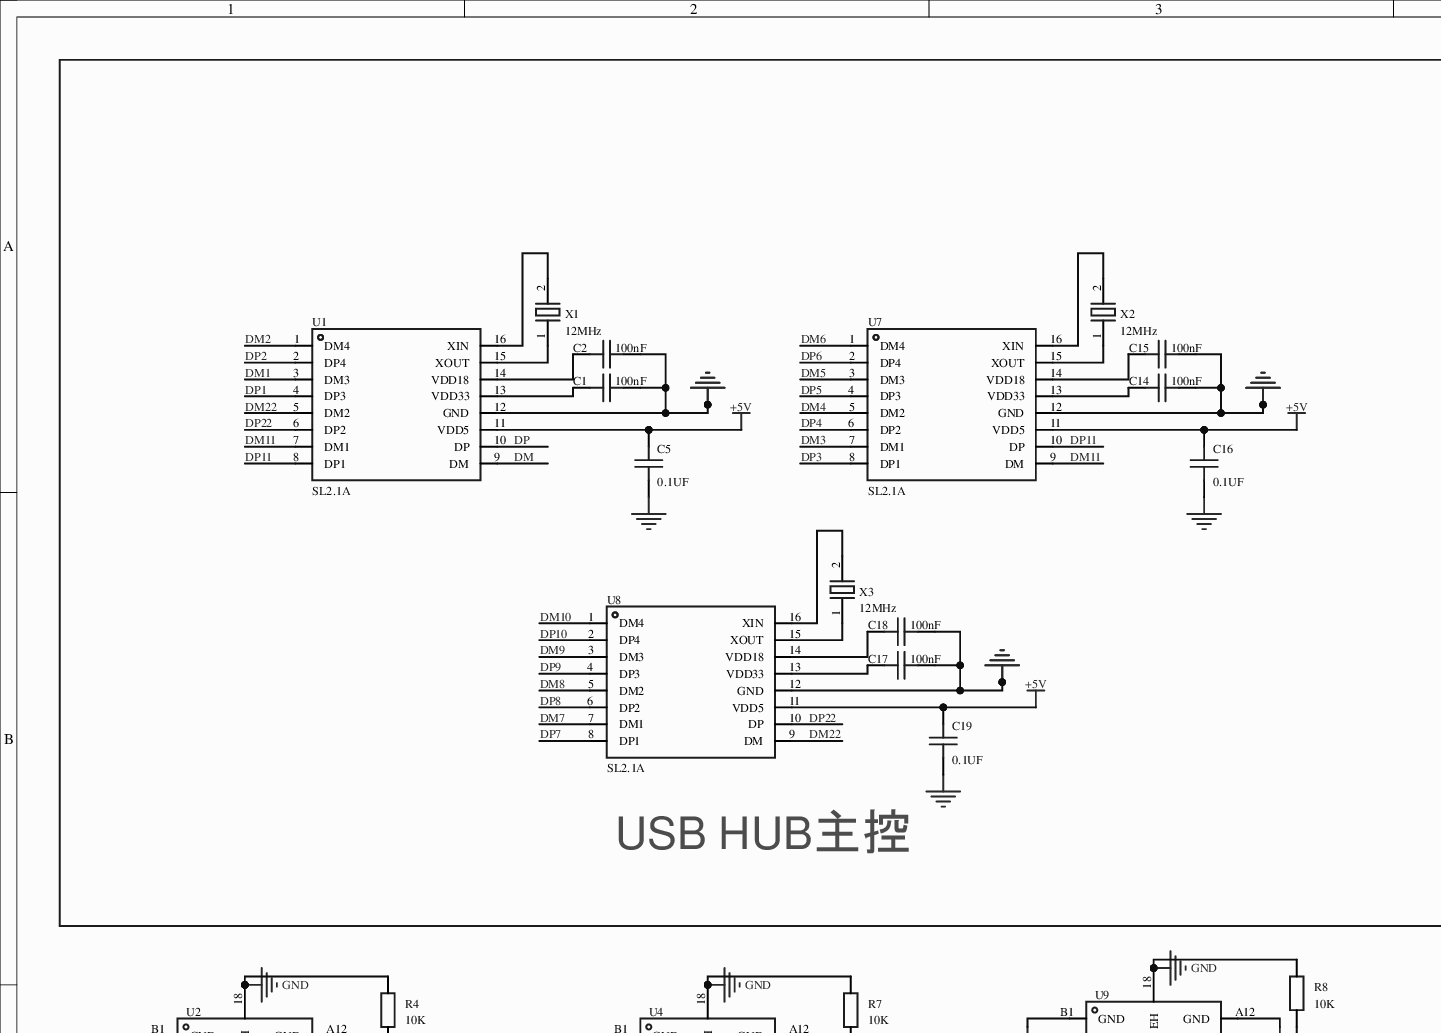
[diagram p0: MISC51596-3.schdoc, top left]
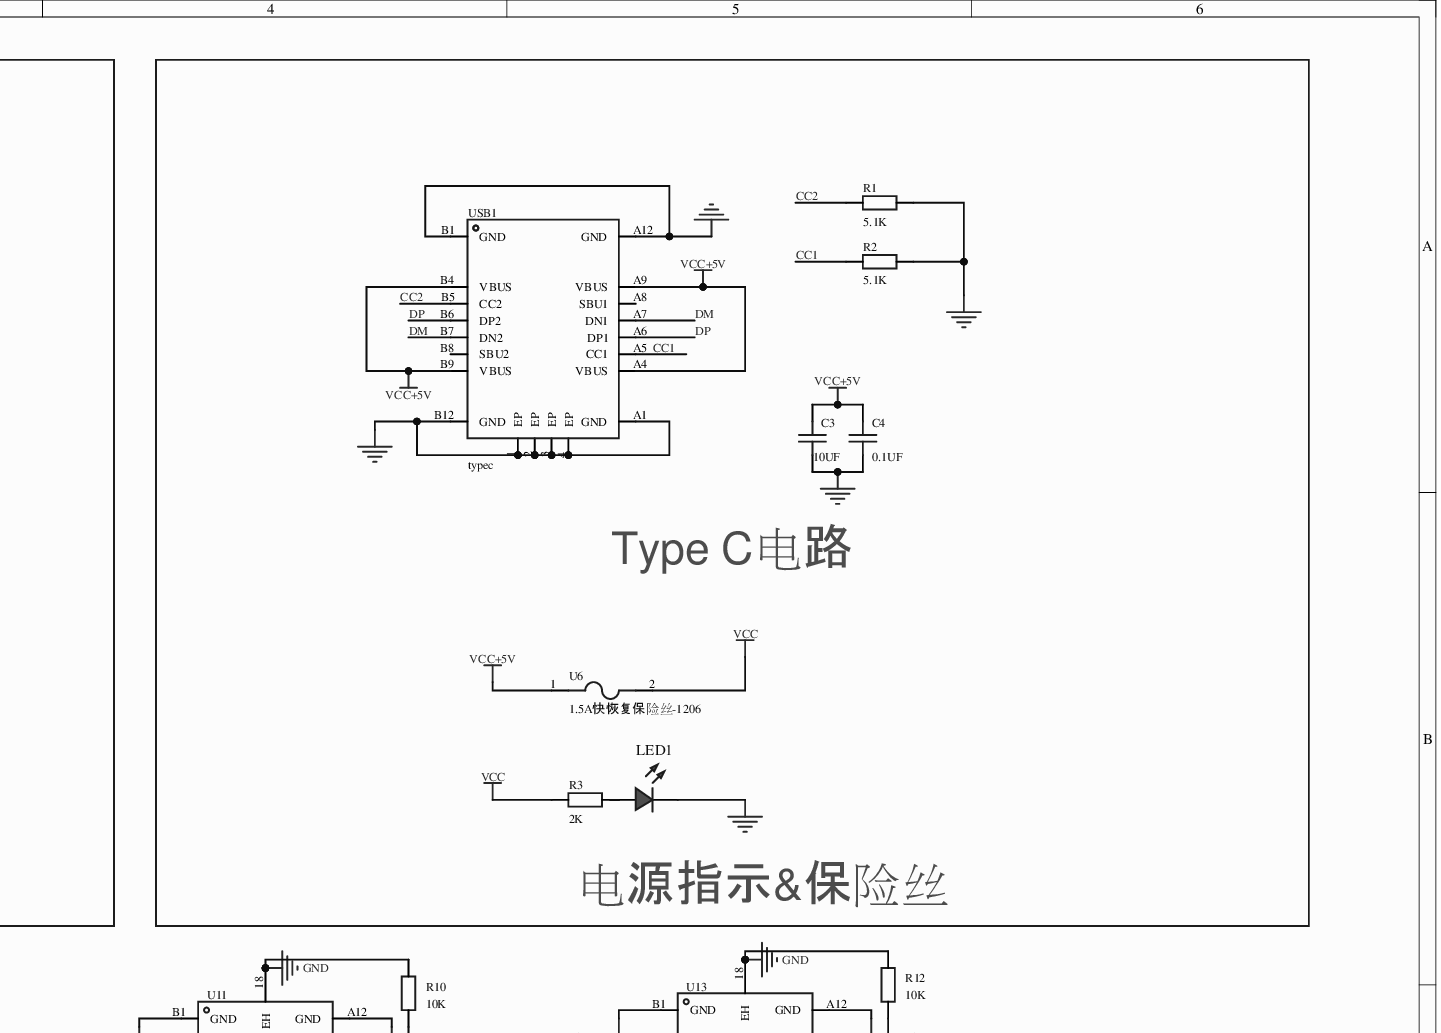
[diagram p1: MISC51596-3.schdoc, top right]
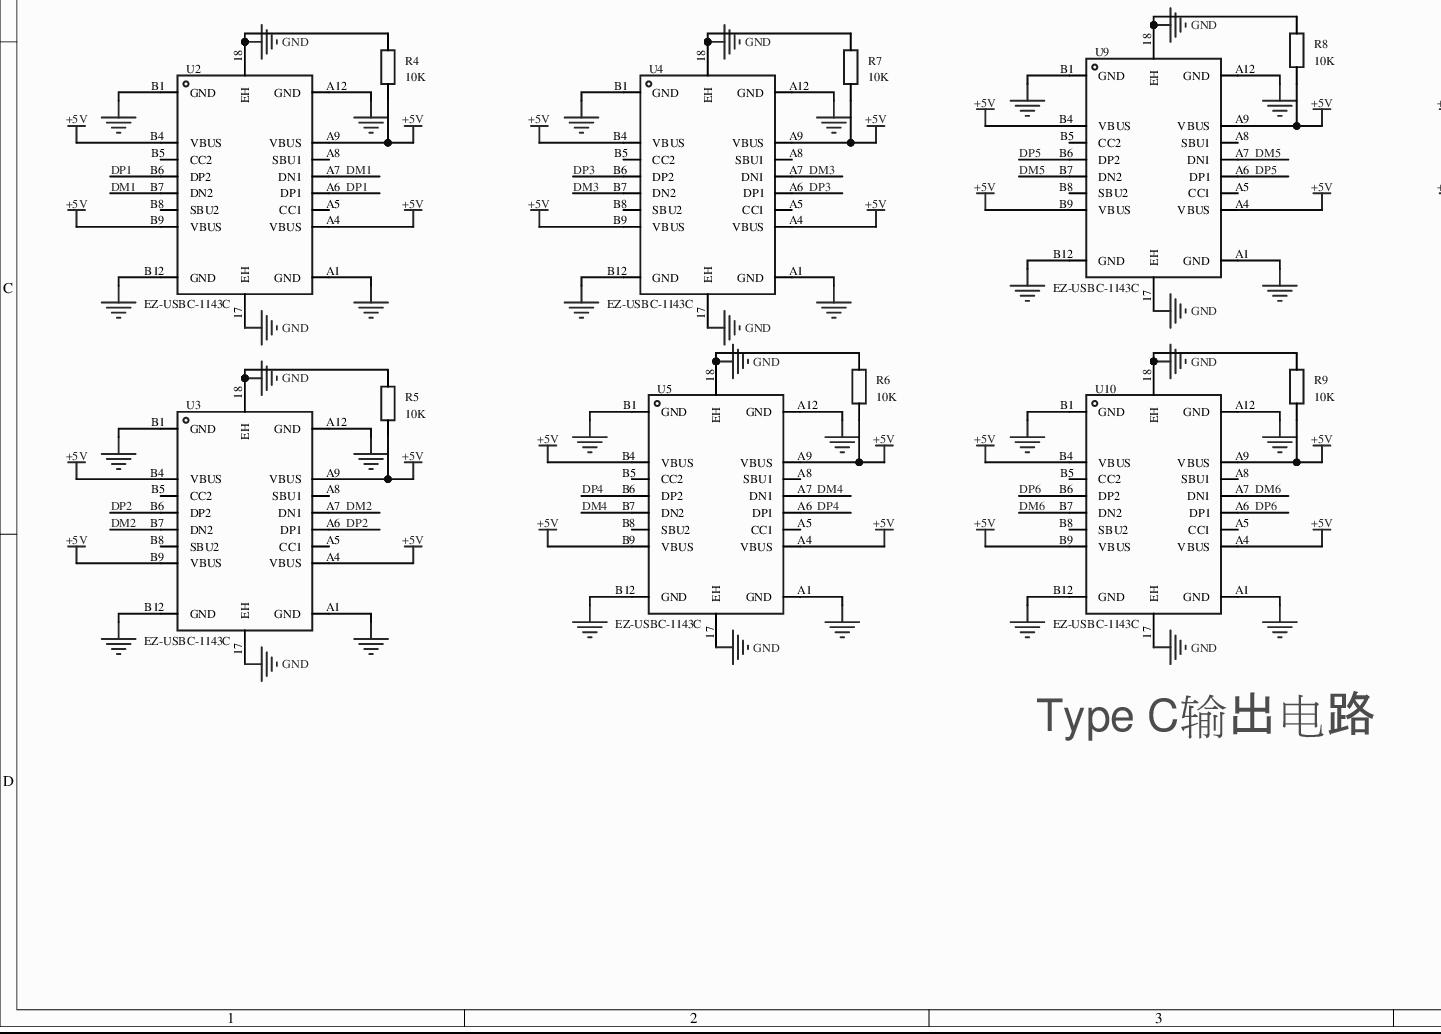
[diagram p2: MISC51596-3.schdoc, bottom left]
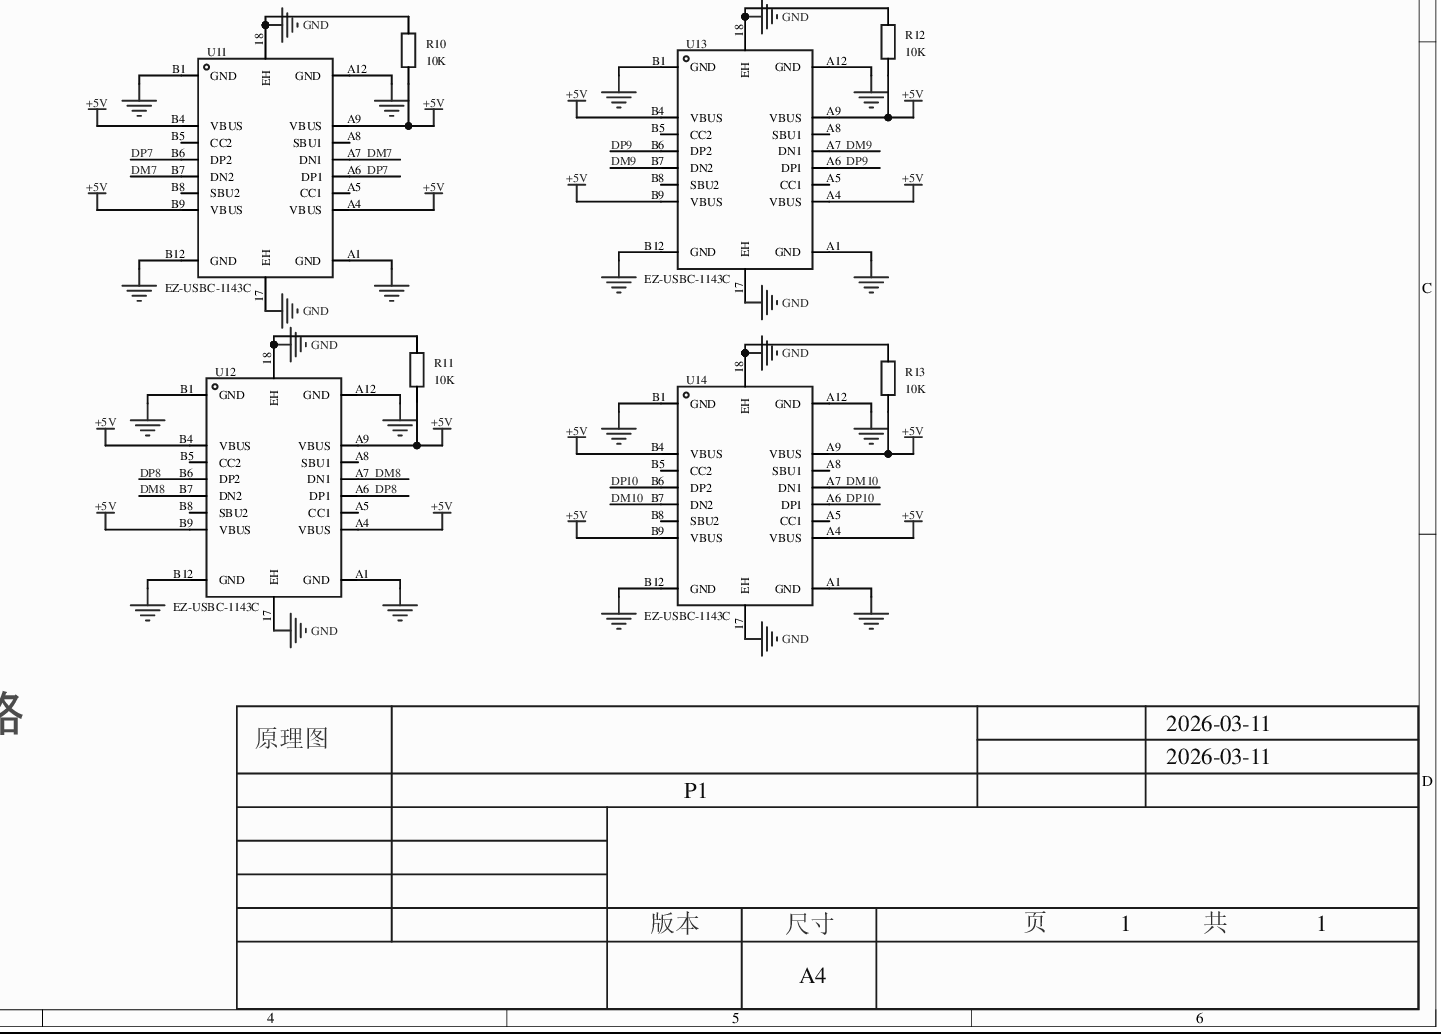
[diagram p3: MISC51596-3.schdoc, bottom right]
# Altium project MISC51596-2.PrjPcb
1 sheet, 43 parts. Net scope: global (net labels, ports and power ports of the same name join across sheets).
Board file: MISC51596.pcbdoc

## Sheet MISC51596-3.schdoc
size 420 x 297 mm; Version: V1.0; @Project Name: MISC51596; @Page Count: 1; @Update Date: 2026-03-11; @Create Date: 2026-03-11; @Schematic Name: MISC51596; @Page No: 1

### Parts
C1  100nF  [C0805]
C2  100nF  [C0805]
C3  10UF  [C0805]
C4  0.1UF  [C0805]
C5  0.1UF  [C0805]
C14  100nF  [C0805]
C15  100nF  [C0805]
C16  0.1UF  [C0805]
C17  100nF  [C0805]
C18  100nF  [C0805]
C19  0.1UF  [C0805]
LED1  (no value)  [LED_0805]
R1  5.1K  [R0805]
R2  5.1K  [R0805]
R3  2K  [R0805]
R4  10K  [R0603]
R5  10K  [R0603]
R6  10K  [R0603]
R7  10K  [R0603]
R8  10K  [R0603]
R9  10K  [R0603]
R10  10K  [R0603]
R11  10K  [R0603]
R12  10K  [R0603]
R13  10K  [R0603]
U1  SL2.1A  [SOP-16_L10.0-W3.9-P1.27-LS6.0-BL]
U2  EZ-USBC-1143C  [USB-SMD_EZ-USBC-1143C]
U3  EZ-USBC-1143C  [USB-SMD_EZ-USBC-1143C]
U4  EZ-USBC-1143C  [USB-SMD_EZ-USBC-1143C]
U5  EZ-USBC-1143C  [USB-SMD_EZ-USBC-1143C]
U6  1.5A快恢复保险丝-1206  [F1206]
U7  SL2.1A  [SOP-16_L10.0-W3.9-P1.27-LS6.0-BL]
U8  SL2.1A  [SOP-16_L10.0-W3.9-P1.27-LS6.0-BL]
U9  EZ-USBC-1143C  [USB-SMD_EZ-USBC-1143C]
U10  EZ-USBC-1143C  [USB-SMD_EZ-USBC-1143C]
U11  EZ-USBC-1143C  [USB-SMD_EZ-USBC-1143C]
U12  EZ-USBC-1143C  [USB-SMD_EZ-USBC-1143C]
U13  EZ-USBC-1143C  [USB-SMD_EZ-USBC-1143C]
U14  EZ-USBC-1143C  [USB-SMD_EZ-USBC-1143C]
USB1  typec  [USB-C-SMD_KH-TYPE-C-16P]
X1  12MHz  [CRYSTAL-SMD_L11.1-W4.8-LS12.3]
X2  12MHz  [CRYSTAL-SMD_L11.1-W4.8-LS12.3]
X3  12MHz  [CRYSTAL-SMD_L11.1-W4.8-LS12.3]

### Blocks framed on the sheet
USB HUB主控: C1 C2 C5 C14-C19 U1 U7 U8 X1-X3

### Nets
+5V: C5.2 C16.2 C19.2 R4.1 R5.1 R6.1 R7.1 R8.1 R9.1 R10.1 R11.1 R12.1 R13.1 U1.11(VDD5) U2.A4(VBUS) U2.A9(VBUS) U2.B4(VBUS) U2.B9(VBUS) U3.A4(VBUS) U3.A9(VBUS) U3.B4(VBUS) U3.B9(VBUS) U4.A4(VBUS) U4.A9(VBUS) U4.B4(VBUS) U4.B9(VBUS) U5.A4(VBUS) U5.A9(VBUS) U5.B4(VBUS) U5.B9(VBUS) U7.11(VDD5) U8.11(VDD5) U9.A4(VBUS) U9.A9(VBUS) U9.B4(VBUS) U9.B9(VBUS) U10.A4(VBUS) U10.A9(VBUS) U10.B4(VBUS) U10.B9(VBUS) U11.A4(VBUS) U11.A9(VBUS) U11.B4(VBUS) U11.B9(VBUS) U12.A4(VBUS) U12.A9(VBUS) U12.B4(VBUS) U12.B9(VBUS) U13.A4(VBUS) U13.A9(VBUS) U13.B4(VBUS) U13.B9(VBUS) U14.A4(VBUS) U14.A9(VBUS) U14.B4(VBUS) U14.B9(VBUS)
GND: C1.2 C2.2 C3.1 C4.1 C5.1 C14.2 C15.2 C16.1 C17.2 C18.2 C19.1 LED1.1(C) R1.2 R2.2 R4.2 R5.2 R6.2 R7.2 R8.2 R9.2 R10.2 R11.2 R12.2 R13.2 U1.12(GND) U2.17(EH) U2.18(EH) U2.A1(GND) U2.A12(GND) U2.B1(GND) U2.B12(GND) U3.17(EH) U3.18(EH) U3.A1(GND) U3.A12(GND) U3.B1(GND) U3.B12(GND) U4.17(EH) U4.18(EH) U4.A1(GND) U4.A12(GND) U4.B1(GND) U4.B12(GND) U5.17(EH) U5.18(EH) U5.A1(GND) U5.A12(GND) U5.B1(GND) U5.B12(GND) U7.12(GND) U8.12(GND) U9.17(EH) U9.18(EH) U9.A1(GND) U9.A12(GND) U9.B1(GND) U9.B12(GND) U10.17(EH) U10.18(EH) U10.A1(GND) U10.A12(GND) U10.B1(GND) U10.B12(GND) U11.17(EH) U11.18(EH) U11.A1(GND) U11.A12(GND) U11.B1(GND) U11.B12(GND) U12.17(EH) U12.18(EH) U12.A1(GND) U12.A12(GND) U12.B1(GND) U12.B12(GND) U13.17(EH) U13.18(EH) U13.A1(GND) U13.A12(GND) U13.B1(GND) U13.B12(GND) U14.17(EH) U14.18(EH) U14.A1(GND) U14.A12(GND) U14.B1(GND) U14.B12(GND) USB1.1(EP) USB1.2(EP) USB1.3(EP) USB1.4(EP) USB1.A1(GND) USB1.A12(GND) USB1.B1(GND) USB1.B12(GND)
VCC: R3.2 U6.2
VCC+5V: C3.2 C4.2 U6.1 USB1.A4(VBUS) USB1.A9(VBUS) USB1.B4(VBUS) USB1.B9(VBUS)
CC1: R2.1 USB1.A5(CC1)
CC2: R1.1 USB1.B5(CC2)
DM: U1.9(DM) USB1.A7(DN1) USB1.B7(DN2)
DM1: U1.3(DM3) U2.A7(DN1) U2.B7(DN2)
DM2: U1.1(DM4) U3.A7(DN1) U3.B7(DN2)
DM3: U4.A7(DN1) U4.B7(DN2) U7.7(DM1)
DM4: U5.A7(DN1) U5.B7(DN2) U7.5(DM2)
DM5: U7.3(DM3) U9.A7(DN1) U9.B7(DN2)
DM6: U7.1(DM4) U10.A7(DN1) U10.B7(DN2)
DM7: U8.7(DM1) U11.A7(DN1) U11.B7(DN2)
DM8: U8.5(DM2) U12.A7(DN1) U12.B7(DN2)
DM9: U8.3(DM3) U13.A7(DN1) U13.B7(DN2)
DM10: U8.1(DM4) U14.A7(DN1) U14.B7(DN2)
DM11: U1.7(DM1) U7.9(DM)
DM22: U1.5(DM2) U8.9(DM)
DP: U1.10(DP) USB1.A6(DP1) USB1.B6(DP2)
DP1: U1.4(DP3) U2.A6(DP1) U2.B6(DP2)
DP2: U1.2(DP4) U3.A6(DP1) U3.B6(DP2)
DP3: U4.A6(DP1) U4.B6(DP2) U7.8(DP1)
DP4: U5.A6(DP1) U5.B6(DP2) U7.6(DP2)
DP5: U7.4(DP3) U9.A6(DP1) U9.B6(DP2)
DP6: U7.2(DP4) U10.A6(DP1) U10.B6(DP2)
DP7: U8.8(DP1) U11.A6(DP1) U11.B6(DP2)
DP8: U8.6(DP2) U12.A6(DP1) U12.B6(DP2)
DP9: U8.4(DP3) U13.A6(DP1) U13.B6(DP2)
DP10: U8.2(DP4) U14.A6(DP1) U14.B6(DP2)
DP11: U1.8(DP1) U7.10(DP)
DP22: U1.6(DP2) U8.10(DP)
NetC1_1: C1.1 U1.13(VDD33)
NetC2_1: C2.1 U1.14(VDD18)
NetC14_1: C14.1 U7.13(VDD33)
NetC15_1: C15.1 U7.14(VDD18)
NetC17_1: C17.1 U8.13(VDD33)
NetC18_1: C18.1 U8.14(VDD18)
NetLED1_2: LED1.2(A) R3.1
NetU1_15: U1.15(XOUT) X1.1
NetU1_16: U1.16(XIN) X1.2(GND)
NetU7_15: U7.15(XOUT) X2.1
NetU7_16: U7.16(XIN) X2.2(GND)
NetU8_15: U8.15(XOUT) X3.1
NetU8_16: U8.16(XIN) X3.2(GND)

Not connected (* = marked no-connect by the designer): U2 A5(CC1) A8(SBU1) B5(CC2) B8(SBU2); U3 A5(CC1) A8(SBU1) B5(CC2) B8(SBU2); U4 A5(CC1) A8(SBU1) B5(CC2) B8(SBU2); U5 A5(CC1) A8(SBU1) B5(CC2) B8(SBU2); U9 A5(CC1) A8(SBU1) B5(CC2) B8(SBU2); U10 A5(CC1) A8(SBU1) B5(CC2) B8(SBU2); U11 A5(CC1) A8(SBU1) B5(CC2) B8(SBU2); U12 A5(CC1) A8(SBU1) B5(CC2) B8(SBU2); U13 A5(CC1) A8(SBU1) B5(CC2) B8(SBU2); U14 A5(CC1) A8(SBU1) B5(CC2) B8(SBU2); USB1 A8(SBU1)* B8(SBU2)*

### Notes on the sheet
- Type C电路
- 电源指示&保险丝
- Type C输出电路
- 2026-03-11
- 原理图
- P1
- 版本
- 尺寸
- A4
- 页
- 1
- 共

### Library data of the parts
C1-C5 = CAP_0805: Symbol: CapAcitance; ConvertToPcb: yes; ModelId: 1ba041120af144c991958decab20d241; ModelName: C0805_L2.0-W1.3-H1.3; ModelTransform: 78.74,51.181,0,0,0,0,0,0.0005,0; Device: CAP_0805; AddInBom: yes; Supplier Footprint: 0805; FootprintName: C0805
  C1 C2: Value: 100nF
  C3: Value: 10UF
  C4 C5: Value: 0.1UF
C14-C19 = CAP_0805: Symbol: CapAcitance; 3D Model: 1ba041120af144c991958decab20d241; 3D Model Transform: 78.74,51.181,0,0,0,0,0,0.0005,0; ConvertToPcb: yes; ModelName: C0805_L2.0-W1.3-H1.3; Device: CAP_0805; Supplier Footprint: 0805; AddInBom: yes; FootprintName: C0805
  C14 C15 C17 C18: Value: 100nF
  C16 C19: Value: 0.1UF
LED1 = LED_0805-R: Symbol: LED_R; Convert to PCB: yes; 3D Model: 33fb9fca58e84f37a403ebeef4c28b77; 3D Model Transform: 78.7,49.1,39.3,0,0,0,0,0,0; ModelName: LED-0805_R; Device: LED_0805-R; Add into BOM: yes; Supplier Footprint: 0805; FootprintName: LED_0805
R1-R3 = Res_0805: Symbol: 电阻; ConvertToPcb: yes; ModelId: 37a81e68749a4138bd2dfa6897b24b85; ModelName: R0805_L2.0-W1.3-H0.6; ModelTransform: 78.74,51.181,0,0,0,0,0,-0.0005,0; Device: Res_0805; AddInBom: yes; Supplier Footprint: 0805; FootprintName: R0805
  R1 R2: Value: 5.1K
  R3: Value: 2K
R4-R13 = Res_0603: Symbol: 电阻; ConvertToPcb: yes; ModelId: fc143cca1e79419f9cd78b61e9279f080819f05c4eef4c71ace90d822a990e87; ModelTransform: 31.8897,63.7794,0,90,0,0,0,0,0; Device: Res_0603; AddInBom: yes; Supplier Footprint: 0603; FootprintName: R0603; ModelName: R0603; Value: 10K
U1 = SL2.1A: 应用功能:集线器;接口协议:-;; Manufacturer: CoreChips(和芯润德); AddInBom: yes; ModelId: 3361a6792abf4a8f8fbca4f1924a67ee; ModelName: SOP-16_L9.9-W3.9-H1.5-LS6.0-P1.27; ModelTransform: 240.39054,393.7,0,90,0,0,0,0,0; Applications Function: 集线器; Symbol: SL2.1A; Device: SL2.1A; LCSC Part Name: SL2.1A USB2.0 HUB 控制器集成电路; SupplierPart: C192893; ManufacturerPart: SL2.1A; Supplier Footprint: SOP-16; JLCPCB Part Class: 扩展库; Datasheet: https://atta.szlcsc.com/upload/public/pdf/source/20180522/C192893_624110D24898D57AAC785E3DF98EA862.pdf; Supplier: LCSC; ConvertToPcb: yes; FootprintName: SOP-16_L10.0-W3.9-P1.27-LS6.0-BL; Protocol: -
U2-U5 U9-U14 = EZ-USBC-1143C: AddInBom: yes; Symbol: EZ-USBC-1143C; Device: EZ-USBC-1143C; LCSC Part Name: EZ-USBC-1143C; SupplierPart: C9900106369; ManufacturerPart: EZ-USBC-1143C; Supplier Footprint: TYPE-C; JLCPCB Part Class: Extended Part; Supplier: LCSC; ConvertToPcb: yes; FootprintName: USB-SMD_EZ-USBC-1143C
U6 = 1.5A快恢复保险丝-1206: AddInBom: yes; ModelId: f1628daad26847a79b887277a2bc8541; ModelName: F1206_L3.2-W1.7-H0.6; ModelTransform: 125.984,66.929,0,0,0,0,0,0,0; Symbol: 1.5A快恢复保险丝-1206; Device: 1.5A快恢复保险丝-1206; LCSC Part Name: 1.5A快恢复保险丝-1206; SupplierPart: C9900012139; ManufacturerPart: 1.5A快恢复保险丝-1206; Supplier Footprint: F1206; JLCPCB Part Class: 扩展库; Supplier: LCSC; ConvertToPcb: yes; FootprintName: F1206
U7 U8 = SL2.1A: 应用功能:集线器;接口协议:-;; Manufacturer: CoreChips(和芯润德); 3D Model: 3361a6792abf4a8f8fbca4f1924a67ee; 3D Model Transform: 240.39054,393.7,0,90,0,0,0,0,0; Applications Function: 集线器; AddInBom: yes; ModelName: SOP-16_L9.9-W3.9-H1.5-LS6.0-P1.27; Symbol: SL2.1A; Device: SL2.1A; LCSC Part Name: SL2.1A USB2.0 HUB 控制器集成电路; Supplier Part: C192893; Manufacturer Part: SL2.1A; Supplier Footprint: SOP-16; JLCPCB Part Class: 扩展库; Datasheet: https://atta.szlcsc.com/upload/public/pdf/source/20180522/C192893_624110D24898D57AAC785E3DF98EA862.pdf; Supplier: LCSC; Protocol: -; ConvertToPcb: yes; FootprintName: SOP-16_L10.0-W3.9-P1.27-LS6.0-BL
USB1 = typec: Symbol: TYPEC_C9900016956; AddInBom: yes; ModelId: f2c381012fbf47e0b76dea5162270f01; ModelTransform: 351.9678,307.48,0,0,0,0,0,-45.275,-43.307; Device: typec; LCSC Part Name: typec; SupplierPart: C9900016956; ManufacturerPart: typec; Supplier Footprint: typec 12p; JLCPCB Part Class: 扩展库; Supplier: LCSC; ConvertToPcb: yes; FootprintName: USB-C-SMD_KH-TYPE-C-16P; ModelName: USB-C-SMD_KH-TYPE-C-16P
X1 = 9AT12000201060C3: 晶振类型:贴片晶振;频率:12MHz;常温频差:±10ppm;外接负载电容:20pF;; Manufacturer: JGHC(晶光华); AddInBom: yes; ModelId: 5e1ead0cf76448b7a4ec480b96b3d6f4; ModelTransform: 484.251,190.1571,0,0,0,0,0,0,0; Crystal Type: 贴片晶振; Normal temperature Frequency Tolerance: ±10ppm; External load capacitor: 20pF; Equivalent Series Resistance (ESR): 60Ω; Symbol: 9AT12000201060C3; Device: 9AT12000201060C3; LCSC Part Name: 12MHz ±10ppm 20pF; SupplierPart: C2715880; ManufacturerPart: 9AT12000201060C3; Supplier Footprint: HC-49S-SMD; JLCPCB Part Class: 扩展库; Datasheet: https://atta.szlcsc.com/upload/public/pdf/source/20210402/C2715880_322A8E636A60333B79E5FA4934B2EA11.pdf; Supplier: LCSC; ConvertToPcb: yes; FootprintName: CRYSTAL-SMD_L11.1-W4.8-LS12.3; ModelName: CRYSTAL-SMD_L11.1-W4.8-LS12.3; Value: 12MHz; Operating Temperature: -40℃~+85℃
X2 X3 = 9AT12000201060C3: 晶振类型:贴片晶振;频率:12MHz;常温频差:±10ppm;外接负载电容:20pF;; Manufacturer: JGHC(晶光华); 3D Model: 5e1ead0cf76448b7a4ec480b96b3d6f4; 3D Model Transform: 484.251,190.1571,0,0,0,0,0,0,0; Crystal Type: 贴片晶振; Normal temperature Frequency Tolerance: ±10ppm; External load capacitor: 20pF; Equivalent Series Resistance (ESR): 60Ω; AddInBom: yes; Symbol: 9AT12000201060C3; Device: 9AT12000201060C3; LCSC Part Name: 12MHz ±10ppm 20pF; Supplier Part: C2715880; Manufacturer Part: 9AT12000201060C3; Supplier Footprint: HC-49S-SMD; JLCPCB Part Class: 扩展库; Datasheet: https://atta.szlcsc.com/upload/public/pdf/source/20210402/C2715880_322A8E636A60333B79E5FA4934B2EA11.pdf; Supplier: LCSC; Value: 12MHz; Operating Temperature: -40℃~+85℃; ConvertToPcb: yes; FootprintName: CRYSTAL-SMD_L11.1-W4.8-LS12.3; ModelName: CRYSTAL-SMD_L11.1-W4.8-LS12.3